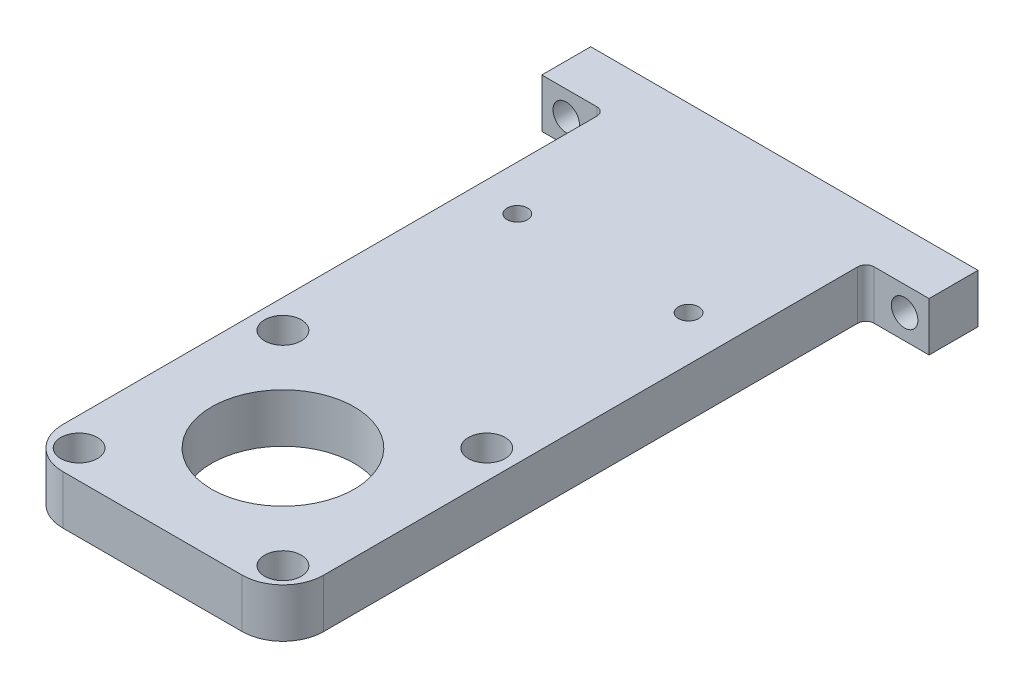
SolidWorks part; units mm, degrees
material "45钢"
ref_plane "前视基准面" through (0, 0, 0) normal (0, 0, 1) x (1, 0, 0)
ref_plane "上视基准面" through (0, 0, 0) normal (0, 1, 0) x (1, 0, 0)
ref_plane "右视基准面" through (0, 0, 0) normal (1, 0, 0) x (0, 0, -1)
sketch "草图1" plane through (0, 0, 0) normal (0, 1, 0) x (1, 0, 0)
  line L0 (0, 0) -> (95, 0)
  line L1 (95, 0) -> (95, -155)
  line L4 (95, -155) -> (0, -155)
  line L5 (0, -155) -> (0, 0)
  dimension "D1" = 95
  dimension "D2" = 155
extrude "凸台-拉伸1" add sketch "草图1" along normal blind 12
hole_wizard "Ø16.0 (16) 直径孔1" positions "草图6" profile "草图5" hole size "Ø16.0" standard "GB"
sketch "草图6" plane through (0, 15, 0) normal (0, 1, 0) x (1, 0, 0)
  line L0 (70, 0) -> (0, 0) construction
  line L2 (35, -31) -> (35, -52) construction
  line L3 (0, -52) -> (70, -52) construction
  point P0 (35, -31)
  dimension "D1" = 31
sketch "草图5" plane through (35, 15, 31) normal (1, 0, 0) x (0, 0, 1)
  line L0 (0, 0) -> (0, 15)
  line L1 (0, 15) -> (8.1, 15)
  line L2 (8.1, 15) -> (8.1, 0)
  line L5 (8.1, 0) -> (0, 0)
  line L11 (0, -6.35) -> (0, 107.95) construction
  dimension "通孔孔直径" = 16.2
  dimension "通孔孔深度" = 15
sketch "草图8" [suppressed] plane through (0, 0, 0) normal (0, -1, 0) x (1, 0, 0)
  line L1 (-59.908, 80.8452) -> (106.3415, 80.8452)
  line L2 (-59.908, 80.8452) -> (-59.908, 14)
  line L3 (-59.908, 14) -> (106.3415, 14)
  line L4 (106.3415, 80.8452) -> (106.3415, 14)
  line L5 (-59.908, 80.8452) -> (106.3415, 14) construction
  line L6 (-59.908, 14) -> (106.3415, 80.8452) construction
  circle A0 centre (35, 31) radius 8.1 construction
  point P0 (23.2167, 47.4226)
  dimension "D1" = 17
extrude "切除-拉伸3" [suppressed] cut sketch "草图8" against normal offset from surface (6 mm away) 9
ref_plane "基准面1" through (47.5, 0, 0) normal (-1, 0, 0) x (0, 0, 1)
sketch "草图9" plane through (0, 12, 0) normal (0, 1, 0) x (1, 0, 0)
  line L0 (95, 0) -> (0, 0) construction
  line L1 (0, -155) -> (15.5, -155)
  line L2 (0, -155) -> (0, -12)
  line L3 (0, -12) -> (15.5, -12)
  line L4 (15.5, -155) -> (15.5, -12)
  line L5 (95, -155) -> (79.5, -155)
  line L6 (95, -155) -> (95, -12)
  line L7 (95, -12) -> (79.5, -12)
  line L8 (79.5, -155) -> (79.5, -12)
  dimension "D1" = 64
  dimension "D2" = 12
extrude "切除-拉伸4" cut sketch "草图9" against normal through all
hole_wizard "Ø6.5 (6.5) 直径孔1" positions "草图10" profile "草图11" hole size "Ø6.5" standard "GB" end condition through all
sketch "草图10" plane through (0, 0, 12) normal (0, 0, 1) x (1, 0, 0)
  line L0 (0, 6) -> (6, 6) construction
  line L1 (0, 0) -> (0, 12) construction
  line L2 (6, 6) -> (89, 6) construction
  line L3 (89, 6) -> (95, 6) construction
  line L4 (95, 0) -> (95, 12) construction
  point P0 (6, 6)
  point P2 (89, 6)
  dimension "D1" = 6
sketch "草图11" plane through (6, 6, 12) normal (1, 0, 0) x (0, -1, 0)
  line L0 (0, 0) -> (0, 12)
  line L1 (0, 12) -> (3.25, 12)
  line L2 (3.25, 12) -> (3.25, 0)
  line L5 (3.25, 0) -> (0, 0)
  line L11 (0, -6.35) -> (0, 107.95) construction
  dimension "通孔孔直径" = 6.5
  dimension "通孔孔深度" = 12
sketch "草图12" plane through (0, 12, 0) normal (0, 1, 0) x (1, 0, 0)
  line L0 (47.5, 0) -> (47.5, -123) construction
  line L1 (95, 0) -> (0, 0) construction
  line L2 (15.5, -155) -> (79.5, -155) construction
  circle A0 centre (47.5, -123) radius 17.5
  dimension "D2" = 35
  dimension "D1" = 32
extrude "切除-拉伸5" cut sketch "草图12" against normal through all
fillet "圆角1" radius 10 2 edges at (15.5, 6, 155) (79.5, 6, 155)
hole_wizard "Ø5.0 (5) 直径孔1" positions "草图13" profile "草图14" hole size "Ø5.0" standard "GB"
sketch "草图13" plane through (0, 0, 0) normal (0, 0, -1) x (-1, 0, 0)
  line L0 (-47.5, 12) -> (-47.5, -2.6375) construction
  line L1 (-95, 12) -> (0, 12) construction
  line L4 (-67.5, 6) -> (-27.5, 6) construction
  line L5 (-27.5, 6) -> (0, 6) construction
  line L6 (0, 12) -> (0, 0) construction
  point P0 (-67.5, 6)
  point P2 (-27.5, 6)
  dimension "D1" = 40
sketch "草图14" plane through (67.5, 6, 0) normal (1, 0, 0) x (0, 1, 0)
  line L0 (0, 0) -> (0, 11.5022)
  line L1 (0, 11.5022) -> (2.5, 10)
  line L2 (2.5, 10) -> (2.5, 0)
  line L5 (2.5, 0) -> (0, 0)
  line L10 (0, 11.5022) -> (-2.5, 10) construction
  line L11 (0, -6.35) -> (0, 107.95) construction
  dimension "孔直径" = 5
  dimension "孔深度" = 10
  dimension "导头角度" = 118
fillet "圆角2" radius 2 2 edges at (15.5, 6, 12) (79.5, 6, 12)
hole_wizard "M6 螺纹孔2" positions "草图23" profile "草图24" tap size "M6" standard "GB" end condition through all
sketch "草图23" plane through (0, 0, 0) normal (0, -1, 0) x (-1, 0, 0)
  line L1 (-47.5, -123) -> (-47.5, 40.9344) construction
  point P8 (-68.5, -44.5)
  point P16 (-26.5, -44.5)
sketch "草图24" plane through (68.5, 0, 44.5) normal (1, 0, 0) x (0, 0, -1)
  line L0 (0, 0) -> (0, 12)
  line L1 (0, 12) -> (2.5, 12)
  line L2 (2.5, 12) -> (2.5, 0)
  line L5 (2.5, 0) -> (0, 0)
  line L11 (0, -6.35) -> (0, 107.95) construction
  dimension "通孔螺纹孔钻头直径" = 5
  dimension "通孔螺纹孔钻头深度" = 12
cosmetic thread "孔螺蚊线2" parameters "D2"=6
cosmetic thread "孔螺蚊线3" parameters "D2"=6
hole_wizard "大小mm 暗销孔1" positions "草图25" profile "草图26" hole size "Ø8.0" standard "GB" end condition through all
sketch "草图25" plane through (0, 0, 0) normal (0, -1, 0) x (-1, 0, 0)
  point P0 (-72.5, -98)
  point P3 (-72.5, -148)
  point P6 (-22.5, -148)
  point P9 (-22.5, -98)
sketch "草图26" plane through (72.5, 0, 98) normal (1, 0, 0) x (0, 0, -1)
  line L0 (0, 0) -> (0, 12)
  line L1 (0, 12) -> (4.5, 12)
  line L2 (4.5, 12) -> (4.5, 0)
  line L5 (4.5, 0) -> (0, 0)
  line L11 (0, -6.35) -> (0, 107.95) construction
  dimension "通孔孔直径" = 9
  dimension "通孔孔深度" = 12
